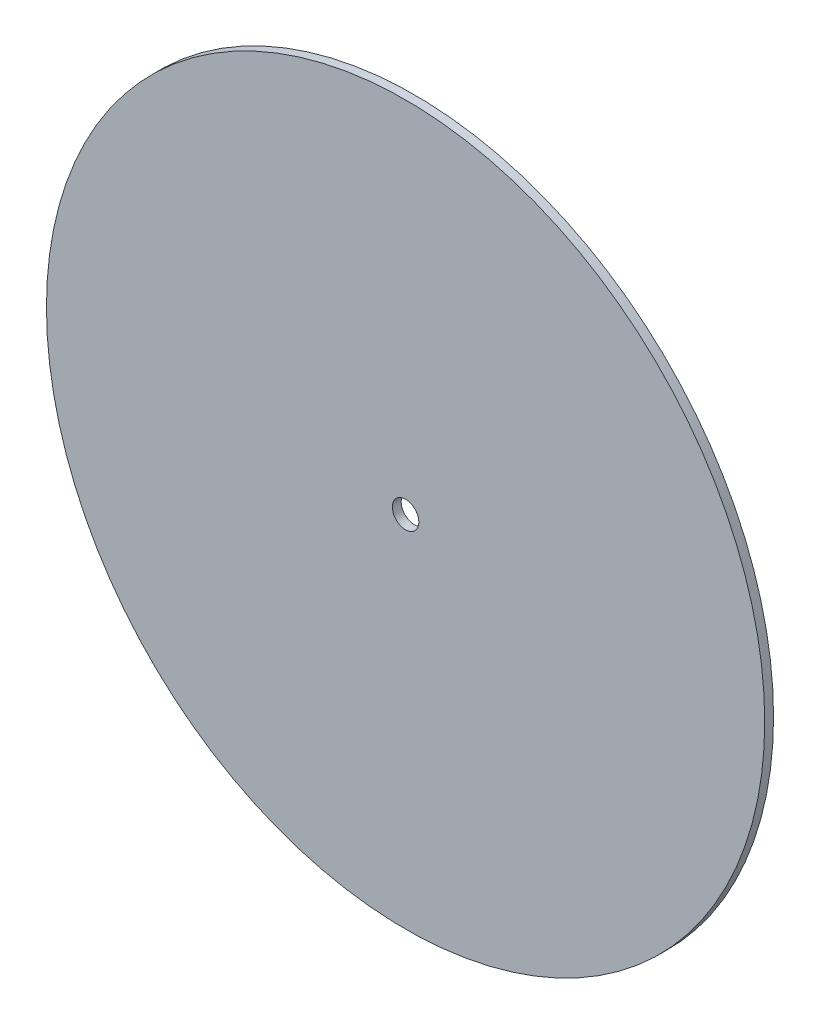
from build123d import *

# Parameters (mm, degrees)
SKETCH_1_R      = 122.25
SKETCH_1_R_2    = 4.5
EXTRUDE_1_DEPTH = 3


with BuildPart() as part:
    # 草图1 → 凸台-拉伸1 (new body)
    with BuildSketch(Plane.XY):
        Circle(SKETCH_1_R)
        Circle(SKETCH_1_R_2, mode=Mode.SUBTRACT)
    extrude(amount=EXTRUDE_1_DEPTH)


solid = part.part
